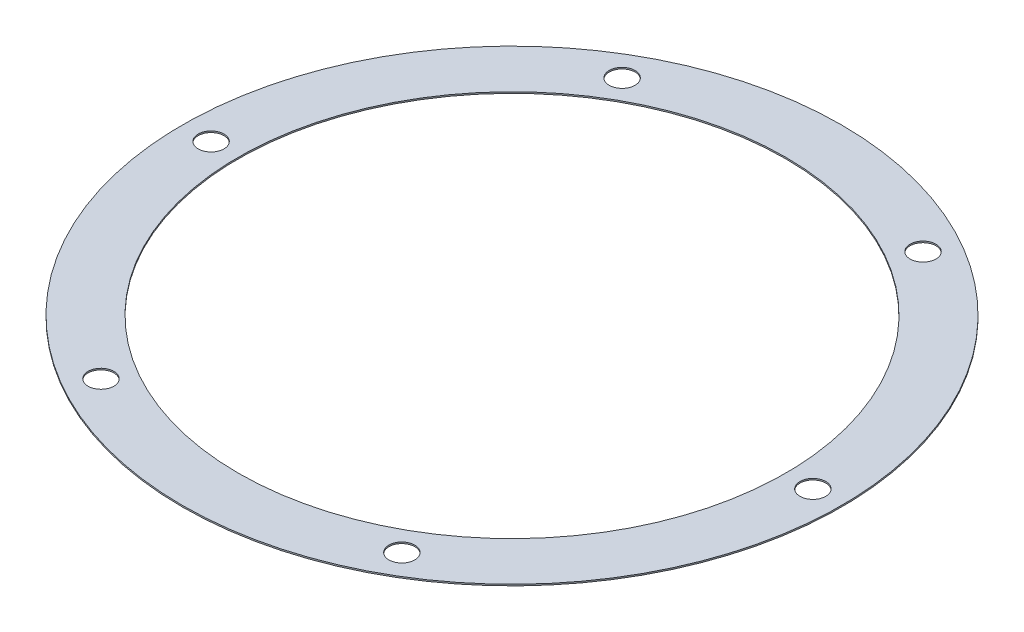
from build123d import *

# Parameters (mm, degrees)
SKETCH1_R           = 230
SKETCH1_R_2         = 191
BOSS_EXTRUDE1_DEPTH = 0.5
SKETCH2_R           = 9
CUT_EXTRUDE2_DEPTH  = 0.5
CIRPATTERN1_COUNT   = 6


with BuildPart() as part:
    # Sketch1 → Boss-Extrude1 (new, symmetric)
    with BuildSketch(Plane(origin=(0, 0, 0), x_dir=(1, 0, 0), z_dir=(0, 1, 0))):
        with Locations(Location((0, 0, 0), (0, 0, 270))):
            Circle(SKETCH1_R)
        with Locations(Location((0, 0, 0), (0, 0, 270))):
            Circle(SKETCH1_R_2, mode=Mode.SUBTRACT)
    extrude(amount=BOSS_EXTRUDE1_DEPTH, both=True)

    # Sketch2 → Cut-Extrude2 (cut, symmetric)
    with BuildSketch(Plane(origin=(0, 0, 0), x_dir=(1, 0, 0), z_dir=(0, 1, 0))):
        with Locations(Location((-210, 0, 0), (0, 0, 270))):
            Circle(SKETCH2_R)
    cut_extrude2 = extrude(amount=CUT_EXTRUDE2_DEPTH, both=True, mode=Mode.SUBTRACT)

    # CirPattern1: Cut-Extrude2 ×6 about axis
    cirpattern1_axis = Axis((0, 0, 0), (0, 1, 0))
    for i in range(1, CIRPATTERN1_COUNT):
        add(cut_extrude2.rotate(cirpattern1_axis, i * 360 / CIRPATTERN1_COUNT), mode=Mode.SUBTRACT)


solid = part.part
